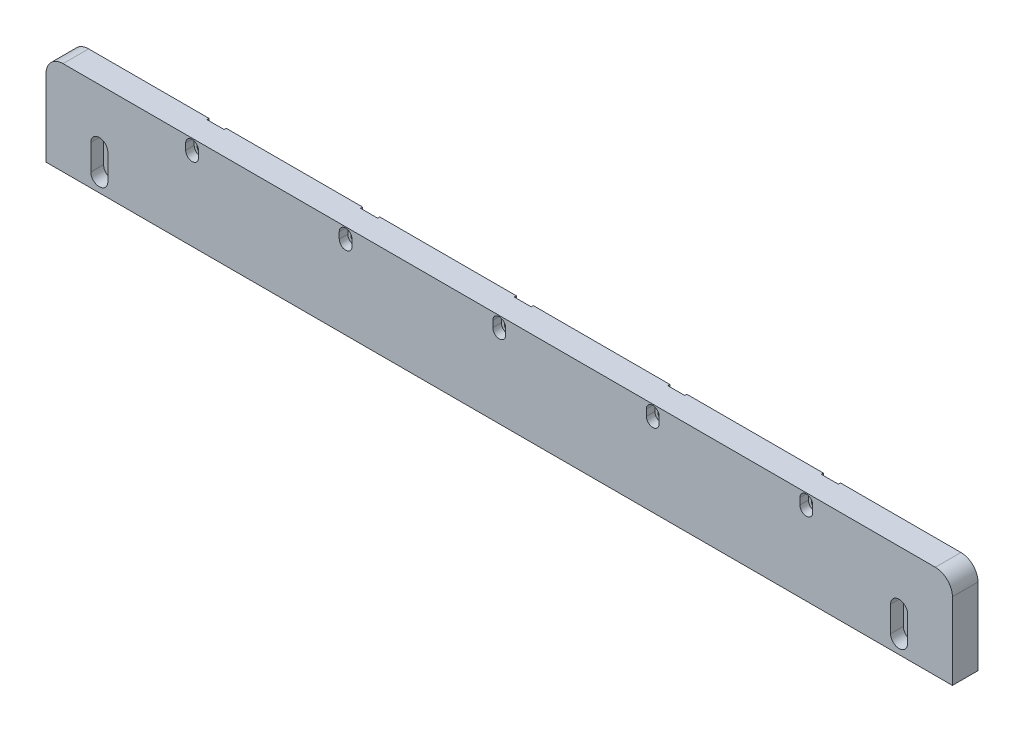
from build123d import *

# Parameters (mm, degrees)
SKETCH_1_W             = 425
SKETCH_1_H             = 44
EXTRUDE_1_DEPTH        = 12
FILLET_1_R             = 8
CUT_EXTRUDE_1_DEPTH    = 6
CUT_EXTRUDE_2_DEPTH    = 214.720027138
SKETCH_4_W             = 8
SKETCH_4_H             = 8.5
CUT_EXTRUDE_3_DEPTH    = 1
CUT_EXTRUDE_4_DEPTH    = 4
CUT_EXTRUDE_5_DEPTH    = 214.785523364
PATTERN_LINEAR_1_COUNT = 5
PATTERN_LINEAR_1_PITCH = 72


with BuildPart() as part:
    # 草图1 → 凸台-拉伸1 (new body)
    with BuildSketch(Plane.XY):
        Rectangle(SKETCH_1_W, SKETCH_1_H)
    extrude(amount=EXTRUDE_1_DEPTH)

    # 圆角1
    fillet_1_edges = [part.edges().sort_by_distance(p)[0] for p in [
        (-212.5, 22, 6),
        (212.5, 22, 6),
    ]]
    fillet(fillet_1_edges, radius=FILLET_1_R)

    # 草图2 → 切除-拉伸1 (cut)
    with BuildSketch(Plane.XY.offset(12)):
        with BuildLine():
            Line((-183.5, -3.5), (-183.5, -15.5))
            ThreePointArc((-183.5, -15.5), (-187.5, -19.5), (-191.5, -15.5))
            Line((-191.5, -15.5), (-191.5, -3.5))
            ThreePointArc((-191.5, -3.5), (-187.5, 0.5), (-183.5, -3.5))
        make_face()
        with BuildLine():
            Line((183.5, -3.5), (183.5, -15.5))
            ThreePointArc((183.5, -15.5), (187.5, -19.5), (191.5, -15.5))
            Line((191.5, -15.5), (191.5, -3.5))
            ThreePointArc((191.5, -3.5), (187.5, 0.5), (183.5, -3.5))
        make_face()
    extrude(amount=-CUT_EXTRUDE_1_DEPTH, mode=Mode.SUBTRACT)

    # 草图3 → 切除-拉伸2 (cut, through all)
    with BuildSketch(Plane.XY.offset(6)):
        with BuildLine():
            Line((-185.5, -3.5), (-185.5, -15.5))
            ThreePointArc((-185.5, -15.5), (-187.5, -17.5), (-189.5, -15.5))
            Line((-189.5, -15.5), (-189.5, -3.5))
            ThreePointArc((-189.5, -3.5), (-187.5, -1.5), (-185.5, -3.5))
        make_face()
        with BuildLine():
            Line((189.5, -3.5), (189.5, -15.5))
            ThreePointArc((189.5, -15.5), (187.5, -17.5), (185.5, -15.5))
            Line((185.5, -15.5), (185.5, -3.5))
            ThreePointArc((185.5, -3.5), (187.5, -1.5), (189.5, -3.5))
        make_face()
    extrude(amount=-CUT_EXTRUDE_2_DEPTH, mode=Mode.SUBTRACT)

    # 草图4 → 切除-拉伸3 (cut)
    with BuildSketch(Plane(origin=(0, 0, 0), x_dir=(-1, 0, 0), z_dir=(0, 0, -1))):
        with Locations((-144, 17.75)):
            Rectangle(SKETCH_4_W, SKETCH_4_H)
        with Locations((-72, 17.75)):
            Rectangle(SKETCH_4_W, SKETCH_4_H)
        with Locations((0, 17.75)):
            Rectangle(SKETCH_4_W, SKETCH_4_H)
        with Locations((72, 17.75)):
            Rectangle(SKETCH_4_W, SKETCH_4_H)
        with Locations((144, 17.75)):
            Rectangle(SKETCH_4_W, SKETCH_4_H)
    extrude(amount=-CUT_EXTRUDE_3_DEPTH, mode=Mode.SUBTRACT)

    # 草图5 → 切除-拉伸4 (cut)
    with BuildSketch(Plane.XY.offset(12)):
        with BuildLine():
            Line((-141, 18.5), (-141, 15.5))
            ThreePointArc((-141, 15.5), (-144, 12.5), (-147, 15.5))
            Line((-147, 15.5), (-147, 18.5))
            ThreePointArc((-147, 18.5), (-144, 21.5), (-141, 18.5))
        make_face()
    cut_extrude_4 = extrude(amount=-CUT_EXTRUDE_4_DEPTH, mode=Mode.SUBTRACT)

    # 草图6 → 切除-拉伸5 (cut, through all)
    with BuildSketch(Plane.XY.offset(8)):
        with BuildLine():
            Line((-142.4, 18.5), (-142.4, 15.5))
            ThreePointArc((-142.4, 15.5), (-144, 13.9), (-145.6, 15.5))
            Line((-145.6, 15.5), (-145.6, 18.5))
            ThreePointArc((-145.6, 18.5), (-144, 20.1), (-142.4, 18.5))
        make_face()
    cut_extrude_5 = extrude(amount=-CUT_EXTRUDE_5_DEPTH, mode=Mode.SUBTRACT)

    # 阵列(线性)1: 切除-拉伸4, 切除-拉伸5 ×5
    with Locations(*[(i * PATTERN_LINEAR_1_PITCH, 0, 0) for i in range(1, PATTERN_LINEAR_1_COUNT)]):
        add(cut_extrude_4, mode=Mode.SUBTRACT)
        add(cut_extrude_5, mode=Mode.SUBTRACT)


solid = part.part
